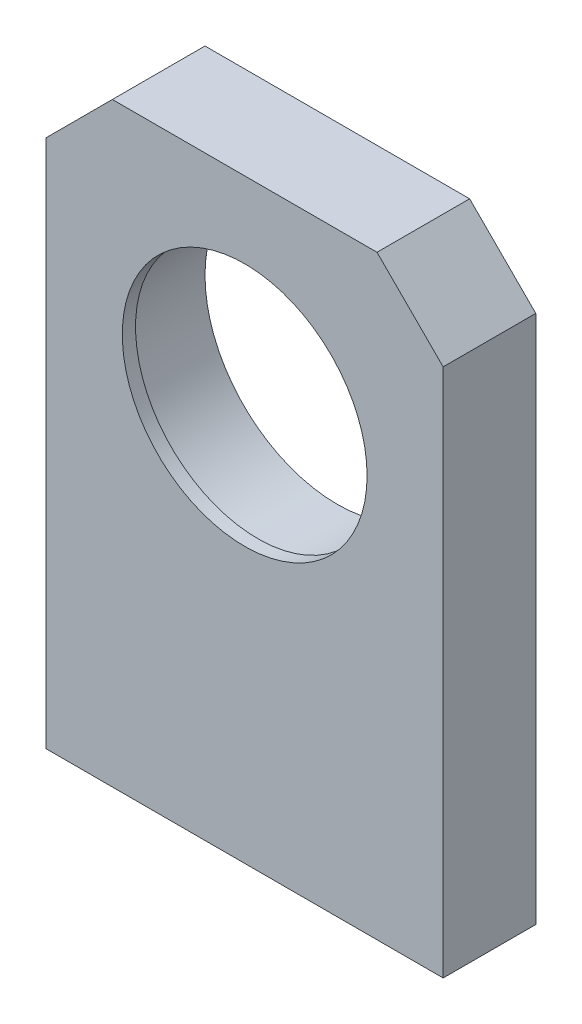
SolidWorks part; units mm, degrees
material "Q235A"
ref_plane "前视基准面" through (0, 0, 0) normal (0, 0, 1) x (1, 0, 0)
ref_plane "上视基准面" through (0, 0, 0) normal (0, 1, 0) x (1, 0, 0)
ref_plane "右视基准面" through (0, 0, 0) normal (1, 0, 0) x (0, 0, -1)
sketch "草图1" plane through (0, 0, 0) normal (0, 0, 1) x (1, 0, 0)
  line L1 (-30, -45) -> (30, -45)
  line L2 (-30, -45) -> (-30, 45)
  line L3 (-30, 45) -> (30, 45)
  line L4 (30, -45) -> (30, 45)
  line L5 (-30, -45) -> (30, 45) construction
  line L6 (-30, 45) -> (30, -45) construction
  circle A0 centre (0, 15) radius 20
  point P0 (0, 0)
  dimension "D1" = 40
  dimension "D2" = 30
  dimension "D3" = 60
  dimension "D4" = 60
extrude "凸台-拉伸1" add sketch "草图1" along normal mid plane 14
sketch "草图2" plane through (0, 0, 7) normal (0, 0, 1) x (1, 0, 0)
  circle A0 centre (0, 15) radius 20 construction
  circle A1 centre (0, 15) radius 20
  circle A2 centre (0, 15) radius 18.5
  dimension "D1" = 37
extrude "凸台-拉伸2" add sketch "草图2" against normal blind 2
chamfer "倒角1" distance 10 angle 45 2 edges at (30, 45, 0) (-30, 45, 0)
hole_wizard "M6 螺纹孔1" positions "3D草图1" profile "草图3" tap size "M6" standard "GB"
sketch3d "3D草图1"
  line L0 (-30, -45, 0) -> (30, -45, 0)
  line L1 (-30, -45, 7) -> (-30, -45, -7) construction
  line L2 (30, -45, 7) -> (30, -45, -7) construction
  point P0 (-24, -45, 0)
  point P2 (24, -45, 0)
sketch "草图3" plane through (-24, -45, 0) normal (1, 0, 0) x (0, 0, -1)
  line L0 (0, 0) -> (0, 15.5022)
  line L1 (0, 15.5022) -> (2.5, 14)
  line L2 (2.5, 14) -> (2.5, 0)
  line L5 (2.5, 0) -> (0, 0)
  line L10 (0, 15.5022) -> (-2.5, 14) construction
  line L11 (0, -6.35) -> (0, 107.95) construction
  dimension "螺纹孔钻头直径" = 5
  dimension "螺纹孔钻头深度" = 14
  dimension "导头角度" = 118
cosmetic thread "孔螺蚊线1"
cosmetic thread "孔螺蚊线2"
equation "\"D2@3D草图1\"=\"D1@3D草图1\""
